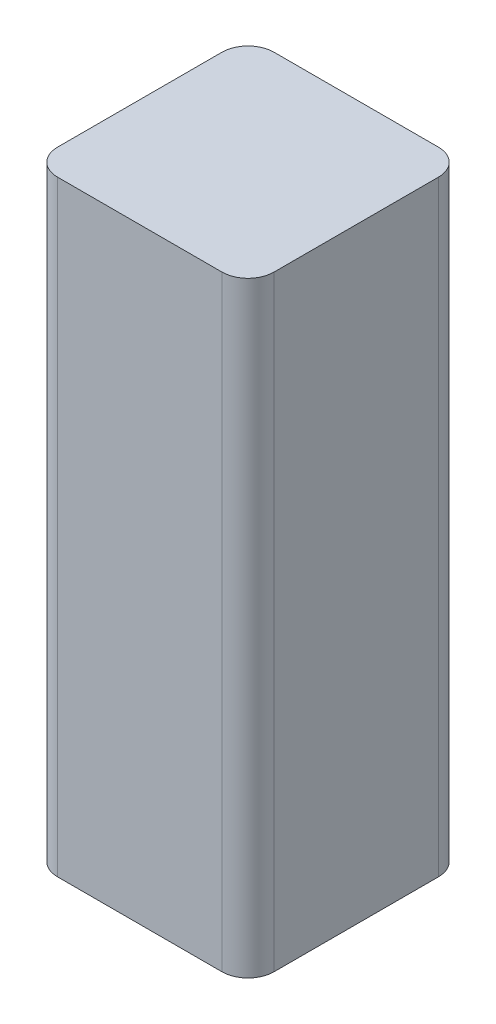
from build123d import *

# Parameters (mm, degrees)
EXTRUDE_1_DEPTH = 140
EXTRUDE_START   = -5
EXTRUDE_2_DEPTH = 5


with BuildPart() as part:
    # 草图1 → 凸台-拉伸1 (new body)
    with BuildSketch(Plane(origin=(0, 0, 0), x_dir=(1, 0, 0), z_dir=(0, 1, 0))):
        with BuildLine():
            Line((-19, -12.278106509), (19, -12.278106509))
            ThreePointArc((19, -12.278106509), (23.242640687, -10.520747196), (25, -6.278106509))
            Line((25, -6.278106509), (25, 31.721893491))
            ThreePointArc((25, 31.721893491), (23.242640687, 35.964534178), (19, 37.721893491))
            Line((19, 37.721893491), (-19, 37.721893491))
            ThreePointArc((-19, 37.721893491), (-23.242640687, 35.964534178), (-25, 31.721893491))
            Line((-25, 31.721893491), (-25, -6.278106509))
            ThreePointArc((-25, -6.278106509), (-23.242640687, -10.520747196), (-19, -12.278106509))
        make_face()
        with BuildLine():
            Line((-19, -7.278106509), (19, -7.278106509))
            ThreePointArc((19, -7.278106509), (19.707106781, -6.98521329), (20, -6.278106509))
            Line((20, -6.278106509), (20, 31.721893491))
            ThreePointArc((20, 31.721893491), (19.707106781, 32.429000272), (19, 32.721893491))
            Line((19, 32.721893491), (-19, 32.721893491))
            ThreePointArc((-19, 32.721893491), (-19.707106781, 32.429000272), (-20, 31.721893491))
            Line((-20, 31.721893491), (-20, -6.278106509))
            ThreePointArc((-20, -6.278106509), (-19.707106781, -6.98521329), (-19, -7.278106509))
        make_face(mode=Mode.SUBTRACT)
    extrude(amount=EXTRUDE_1_DEPTH)

    # 草图2 → 凸台-拉伸2 (add)
    with BuildSketch(Plane(origin=(0, 140, 0), x_dir=(1, 0, 0), z_dir=(0, 1, 0)).offset(EXTRUDE_START)):
        with BuildLine():
            Line((-19, -12.278106509), (19, -12.278106509))
            ThreePointArc((19, -12.278106509), (23.242640687, -10.520747196), (25, -6.278106509))
            Line((25, -6.278106509), (25, 31.721893491))
            ThreePointArc((25, 31.721893491), (23.242640687, 35.964534178), (19, 37.721893491))
            Line((19, 37.721893491), (-19, 37.721893491))
            ThreePointArc((-19, 37.721893491), (-23.242640687, 35.964534178), (-25, 31.721893491))
            Line((-25, 31.721893491), (-25, -6.278106509))
            ThreePointArc((-25, -6.278106509), (-23.242640687, -10.520747196), (-19, -12.278106509))
        make_face()
    extrude(amount=EXTRUDE_2_DEPTH)


solid = part.part
